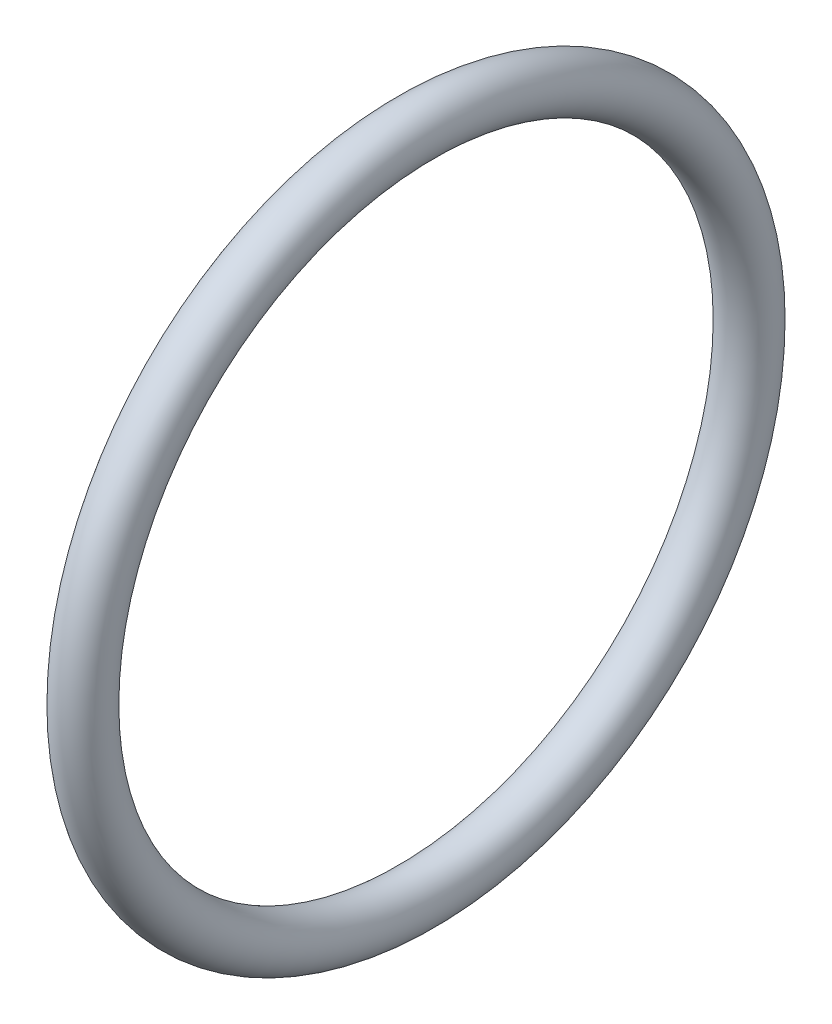
SolidWorks part; units mm, degrees
ref_plane "Front Plane" through (0, 0, 0) normal (0, 0, 1) x (1, 0, 0)
ref_plane "Top Plane" through (0, 0, 0) normal (0, 1, 0) x (1, 0, 0)
ref_plane "Right Plane" through (0, 0, 0) normal (1, 0, 0) x (0, 0, -1)
other "Configuration Table"
sketch "Sketch1" plane through (0, 0, 0) normal (0, 0, 1) x (1, 0, 0)
  line L1 (0, 0) -> (5, 0)
  circle A1 centre (5, 17.35) radius 1.325
  dimension "D2" = 2.65
  dimension "D1" = 17.35
  dimension "D3" = 5
revolve "Revolve1" add sketch "Sketch1" angle 360 about L1
